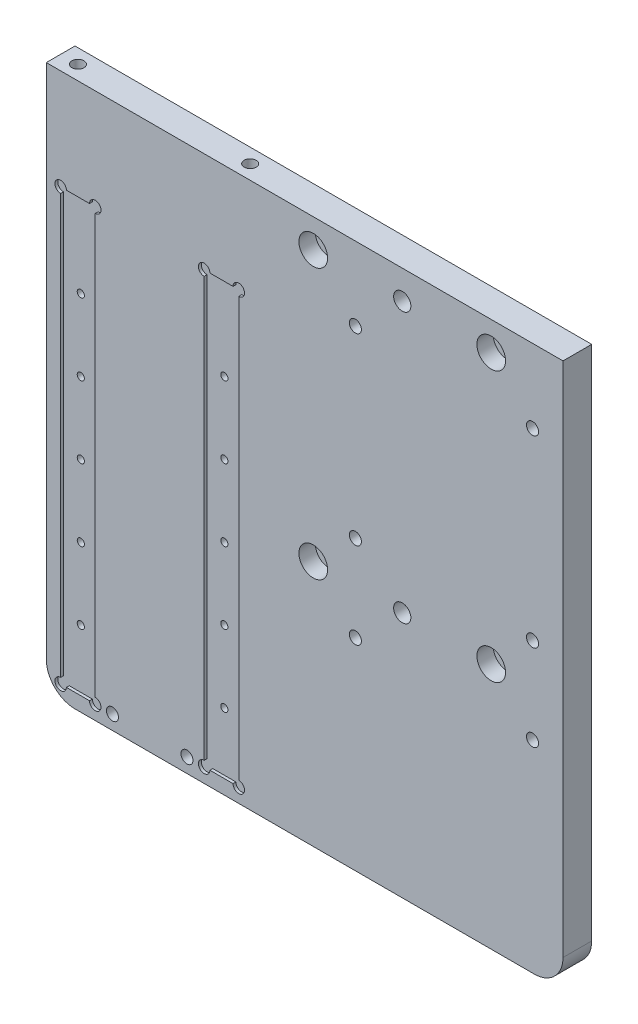
SolidWorks part; units mm, degrees
material "6061铝"
ref_plane "前视基准面" through (0, 0, 0) normal (0, 0, 1) x (1, 0, 0)
ref_plane "上视基准面" through (0, 0, 0) normal (0, 1, 0) x (1, 0, 0)
ref_plane "右视基准面" through (0, 0, 0) normal (1, 0, 0) x (0, 0, -1)
sketch "草图1" plane through (0, 0, 0) normal (0, 0, 1) x (1, 0, 0)
  line L0 (-90, 0) -> (90, 0)
  line L1 (-90, 0) -> (-90, -190)
  line L4 (-90, -190) -> (90, -190)
  line L7 (90, -190) -> (90, 0)
  dimension "D1" = 180
  dimension "D4" = 190
extrude "凸台-拉伸1" add sketch "草图1" along normal blind 10
hole_wizard "打孔尺寸(%根据)开槽圆柱头螺钉的类型1" positions "草图2" profile "草图3" counterbore size "M5" standard "GB" end condition through all
sketch "草图2" plane through (0, 0, 10) normal (0, 0, 1) x (1, 0, 0)
  line L0 (90, 0) -> (-90, 0) construction
  line L1 (90, -190) -> (90, 0) construction
  point P0 (65, -10)
  point P2 (3, -10)
  dimension "D1" = 62
  dimension "D2" = 10
  dimension "D3" = 25
sketch "草图3" plane through (65, -10, 10) normal (1, 0, 0) x (0, -1, 0)
  line L0 (0, 0) -> (0, 10)
  line L1 (0, 10) -> (2.75, 10)
  line L3 (2.75, 10) -> (2.75, 5.7)
  line L4 (2.75, 5.7) -> (5, 5.7)
  line L5 (5, 5.7) -> (5, 0)
  line L7 (5, 0) -> (0, 0)
  line L11 (0, -6.35) -> (0, 107.95) construction
  dimension "通孔孔直径" = 5.5
  dimension "通孔孔深度" = 10
  dimension "柱形沉头孔直径" = 10
  dimension "柱形沉头孔深度" = 5.7
pattern_linear "阵列(线性)1" count 2 spacing 94 along (0, -1, 0) of "打孔尺寸(%根据)开槽圆柱头螺钉的类型1"
sketch "草图4" plane through (0, 0, 10) normal (0, 0, 1) x (1, 0, 0)
  line L0 (-53.975, -22.9657) -> (-53.975, -138.7508) construction
  line L1 (-85, -35) -> (-72.95, -35)
  line L2 (-85, -35) -> (-85, -185)
  line L3 (-85, -185) -> (-72.95, -185)
  line L4 (-72.95, -35) -> (-72.95, -185)
  line L5 (-85, -35) -> (-72.95, -185) construction
  line L6 (-85, -185) -> (-72.95, -35) construction
  line L7 (-22.95, -185) -> (-35, -35) construction
  line L8 (-22.95, -35) -> (-35, -185) construction
  line L9 (-35, -35) -> (-35, -185)
  line L10 (-22.95, -185) -> (-35, -185)
  line L11 (-22.95, -35) -> (-22.95, -185)
  line L12 (-22.95, -35) -> (-35, -35)
  line L14 (-90, 0) -> (-90, -190) construction
  line L15 (90, 0) -> (-90, 0) construction
  point P0 (-78.975, -110)
  point P11 (-28.975, -110)
  dimension "D1" = 12.05
  dimension "D2" = 50
  dimension "D3" = 150
  dimension "D4" = 5
  dimension "D5" = 35
extrude "切除-拉伸1" cut sketch "草图4" against normal blind 1
ref_plane "基准面1" through (-85, -35, 10) normal (-1, 0, 0) x (0, 0, 1)
sketch "草图6" plane through (0, 0, 10) normal (0, 0, 1) x (1, 0, 0)
  line L0 (-85, -31.6862) -> (-85, -38.3138) construction
  line L1 (-72.95, -35) -> (-85, -35) construction
  line L2 (-85, -185) -> (-72.95, -185) construction
  line L3 (-35, -185) -> (-22.95, -185) construction
  circle A0 centre (-72.95, -35) radius 2
  circle A1 centre (-85, -35) radius 2
  circle A2 centre (-85, -185) radius 2
  circle A3 centre (-72.95, -185) radius 2
  circle A4 centre (-35, -185) radius 2
  circle A5 centre (-22.95, -185) radius 2
  circle A6 centre (-35, -35) radius 2
  circle A7 centre (-22.95, -35) radius 2
  dimension "D1" = 4
extrude "切除-拉伸2" cut sketch "草图6" against normal up to surface (1 mm away) up to face at (-78.975, -110, 9)
hole_wizard "M5 螺纹孔1" positions "草图7" profile "草图9" tap size "M5" standard "GB"
sketch "草图7" plane through (0, 0, 0) normal (0, 1, 0) x (1, 0, 0)
  point P0 (-23.975, -5)
  point P3 (-83.975, -5)
sketch "草图9" plane through (-23.975, 0, 5) normal (1, 0, 0) x (0, 0, 1)
  line L0 (0, 0) -> (0, 15.2618)
  line L1 (0, 15.2618) -> (2.1, 14)
  line L2 (2.1, 14) -> (2.1, 0)
  line L5 (2.1, 0) -> (0, 0)
  line L10 (0, 15.2618) -> (-2.1, 14) construction
  line L11 (0, -6.35) -> (0, 107.95) construction
  dimension "螺纹孔钻头直径" = 4.2
  dimension "螺纹孔钻头深度" = 14
  dimension "导头角度" = 118
cosmetic thread "孔螺蚊线3" parameters "D1"=10, "D2"=5
cosmetic thread "孔螺蚊线4" parameters "D1"=10, "D2"=5
fillet "圆角1" radius 10 2 edges at (-90, -190, 5) (90, -190, 5)
hole_wizard "M5 螺纹孔2" positions "草图10" profile "草图11" tap size "M5" standard "GB" end condition through all
sketch "草图10" plane through (0, 0, 10) normal (0, 0, 1) x (1, 0, 0)
  line L0 (-72.95, -183) -> (-72.95, -37) construction
  line L1 (-80, -190) -> (80, -190) construction
  line L3 (-35, -37) -> (-35, -183) construction
  point P0 (-66.95, -185)
  point P2 (-41, -185)
  dimension "D4" = 6
  dimension "D1" = 5
  dimension "D2" = 6
  dimension "D3" = 5
sketch "草图11" plane through (-66.95, -185, 10) normal (1, 0, 0) x (0, -1, 0)
  line L0 (0, 0) -> (0, 10)
  line L1 (0, 10) -> (2.1, 10)
  line L2 (2.1, 10) -> (2.1, 0)
  line L5 (2.1, 0) -> (0, 0)
  line L11 (0, -6.35) -> (0, 107.95) construction
  dimension "通孔螺纹孔钻头直径" = 4.2
  dimension "通孔螺纹孔钻头深度" = 10
cosmetic thread "孔螺蚊线5" parameters "D2"=5
cosmetic thread "孔螺蚊线6" parameters "D2"=5
hole_wizard "M5 螺纹孔3" positions "草图12" profile "草图13" tap size "M5" standard "GB" end condition through all
sketch "草图12" plane through (0, 0, 10) normal (0, 0, 1) x (1, 0, 0)
  point P13 (79.3795, -119.6664)
  point P15 (17.6705, -119.6664)
  point P17 (17.6705, -89.6664)
  point P19 (79.3795, -89.6664)
  point P21 (79.3795, -25.6664)
  point P23 (17.6705, -25.6664)
sketch "草图13" plane through (79.3795, -119.6664, 10) normal (1, 0, 0) x (0, -1, 0)
  line L0 (0, 0) -> (0, 10)
  line L1 (0, 10) -> (2.1, 10)
  line L2 (2.1, 10) -> (2.1, 0)
  line L5 (2.1, 0) -> (0, 0)
  line L11 (0, -6.35) -> (0, 107.95) construction
  dimension "通孔螺纹孔钻头直径" = 4.2
  dimension "通孔螺纹孔钻头深度" = 10
cosmetic thread "孔螺蚊线7" parameters "D2"=5
cosmetic thread "孔螺蚊线8" parameters "D2"=5
cosmetic thread "孔螺蚊线9" parameters "D2"=5
cosmetic thread "孔螺蚊线10" parameters "D2"=5
cosmetic thread "孔螺蚊线11" parameters "D2"=5
cosmetic thread "孔螺蚊线12" parameters "D2"=5
hole_wizard "Ø6.0 (6) 直径孔1" positions "草图14" profile "草图15" hole size "Ø6.0" standard "GB"
sketch "草图14" plane through (0, 0, 10) normal (0, 0, 1) x (1, 0, 0)
  line L1 (3, -10) -> (65, -10) construction
  line L2 (3, -104) -> (65, -104) construction
  point P8 (34, -10)
  point P16 (34, -104)
sketch "草图15" plane through (34, -104, 10) normal (1, 0, 0) x (0, -1, 0)
  line L0 (0, 0) -> (0, 11.8026)
  line L1 (0, 11.8026) -> (3, 10)
  line L2 (3, 10) -> (3, 0)
  line L5 (3, 0) -> (0, 0)
  line L10 (0, 11.8026) -> (-3, 10) construction
  line L11 (0, -6.35) -> (0, 107.95) construction
  dimension "孔直径" = 6
  dimension "孔深度" = 10
  dimension "导头角度" = 118
hole_wizard "M3 螺纹孔1" positions "草图16" profile "草图17" tap size "M3" standard "GB" end condition through all
sketch "草图16" plane through (0, 0, 10) normal (0, 0, 1) x (1, 0, 0)
  point P0 (-28.975, -64.7)
  point P3 (-78.975, -64.7)
  point P6 (-78.975, -89.7)
  point P9 (-78.975, -114.7)
  point P12 (-78.975, -164.7)
  point P15 (-78.975, -139.7)
  point P18 (-28.975, -164.7)
  point P21 (-28.975, -139.7)
  point P24 (-28.975, -114.7)
  point P27 (-28.975, -89.7)
cosmetic thread "孔螺蚊线13" parameters "D2"=3
cosmetic thread "孔螺蚊线14" parameters "D2"=3
cosmetic thread "孔螺蚊线15" parameters "D2"=3
cosmetic thread "孔螺蚊线16" parameters "D2"=3
cosmetic thread "孔螺蚊线17" parameters "D2"=3
cosmetic thread "孔螺蚊线18" parameters "D2"=3
cosmetic thread "孔螺蚊线19" parameters "D2"=3
cosmetic thread "孔螺蚊线20" parameters "D2"=3
cosmetic thread "孔螺蚊线21" parameters "D2"=3
cosmetic thread "孔螺蚊线22" parameters "D2"=3
sketch "草图17" plane through (-28.975, -64.7, 10) normal (1, 0, 0) x (0, -1, 0)
  line L0 (0, 0) -> (0, 10)
  line L1 (0, 10) -> (1.25, 10)
  line L2 (1.25, 10) -> (1.25, 0)
  line L5 (1.25, 0) -> (0, 0)
  line L11 (0, -6.35) -> (0, 107.95) construction
  dimension "通孔螺纹孔钻头直径" = 2.5
  dimension "通孔螺纹孔钻头深度" = 10
